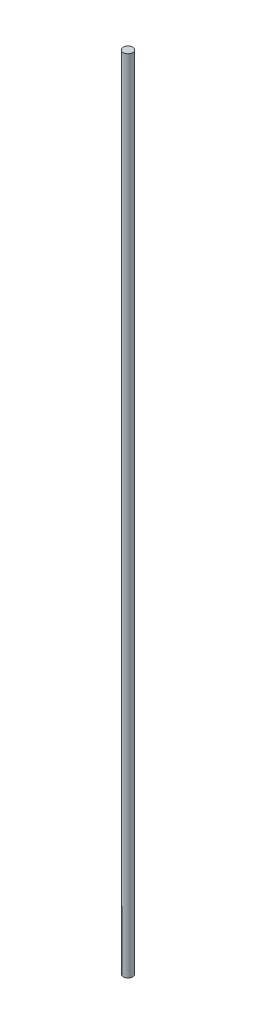
from build123d import *

# Parameters (mm, degrees)
SKETCH1_R           = 2.5
BOSS_EXTRUDE1_DEPTH = 420


with BuildPart() as part:
    # Sketch1 → Boss-Extrude1 (new body)
    with BuildSketch(Plane(origin=(0, 0, 0), x_dir=(1, 0, 0), z_dir=(0, 1, 0))):
        with Locations(Location((0, 0, 0), (0, 0, 270))):
            Circle(SKETCH1_R)
    extrude(amount=BOSS_EXTRUDE1_DEPTH)


solid = part.part
